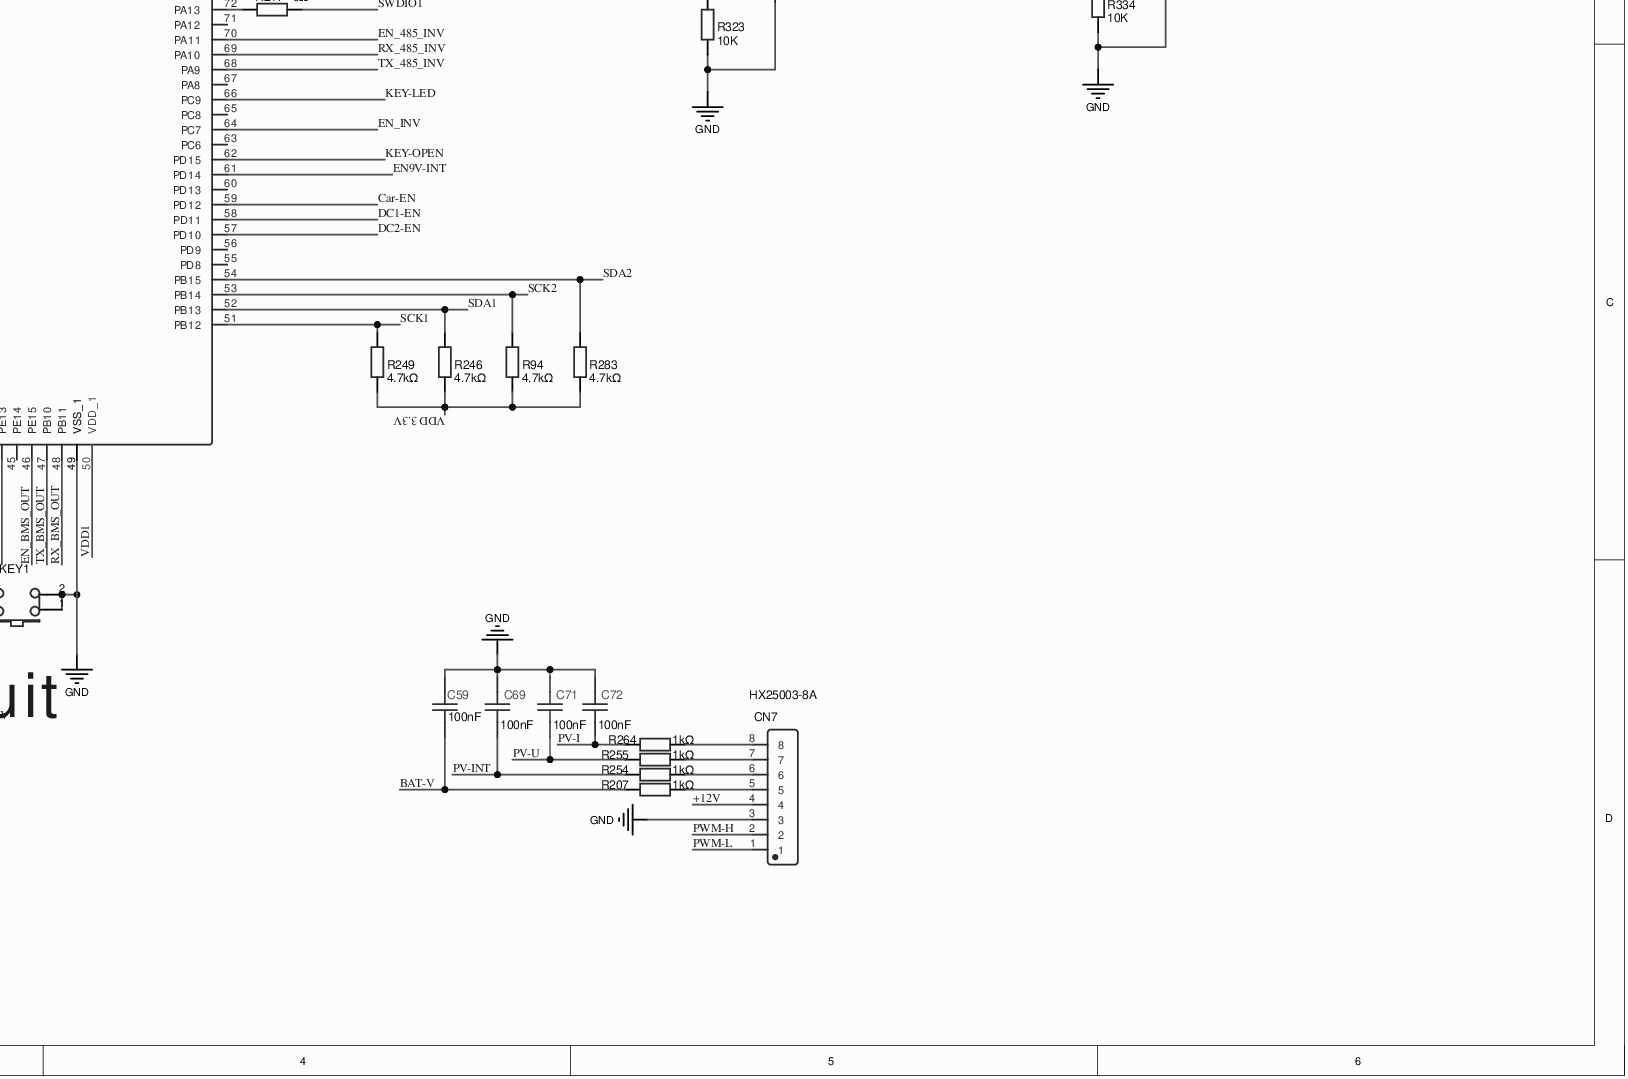
[diagram p0: MISC84402-7.SchDoc, bottom right]
# Altium project MISC84402-4.PrjPcb (part 2 of 7)
## Sheet MISC84402-7.SchDoc (continued)
### Parts (continued)
C9  100nF  [C0603]
C21  100nF  [C0603]
C26  100nF  [C0603]
C32  100nF  [C0603]
C34  100nF  [C0603]
C35  100nF  [C0603]
C39  1nF  [C0603]
C52  100nF  [C0603]
C59  100nF  [C0603]
C69  100nF  [C0603]
C71  100nF  [C0603]
C72  100nF  [C0603]
C73  100nF  [C0603]
C74  100nF  [C0603]
C76  220uF  [CAP-TH_BD6.3-P2.50-D1.0-FD]
C78  100nF  [C0603]
C85  100nF  [C0603]
C87  220uF  [CAP-TH_BD6.3-P2.50-D1.0-FD]
C94  220uF  [CAP-TH_BD6.3-P2.50-D1.0-FD]
C99  100nF  [C0603]
C100  100nF  [C0603]
C126  100nF  [C0603]
C127  100nF  [C0603]
C131  100nF  [C0603]
C133  100nF  [C0603]
C137  100nF  [C0603]
C149  20pF  [C0603]
C152  220uF  [CAP-TH_BD6.3-P2.50-D1.0-FD]
C156  220uF  [CAP-TH_BD6.3-P2.50-D1.0-FD]
C163  20pF  [C0603]
C164  20pF  [C0603]
C167  100nF  [C0603]
C178  4.7uF  [C0805]
CN2  HX25003-4A  [CONN-TH_4P-P2.50_HX25003-4A]
CN7  HX25003-8A  [CONN-TH_8P-P2.50_HX25003-8A]
CN10  HX25003-4A  [CONN-TH_4P-P2.50_HX25003-4A]
D14  SS12  [SMA_L4.3-W2.6-LS5.2-RD]
D46  SMAJ30  [SMA_L4.3-W2.5-LS5.0-BI]
D47  SMAJ30  [SMA_L4.3-W2.5-LS5.0-BI]
KEY1  4-1437565-2  [SW-SMD_4P-L6.0-W6.0-P4.50-LS8.6]  (value not drawn)
KEY2  4-1437565-2  [SW-SMD_4P-L6.0-W6.0-P4.50-LS8.6]  (value not drawn)
KEY3  4-1437565-2  [SW-SMD_4P-L6.0-W6.0-P4.50-LS8.6]  (value not drawn)
KEY4  4-1437565-2  [SW-SMD_4P-L6.0-W6.0-P4.50-LS8.6]  (value not drawn)
KEY5  4-1437565-2  [SW-SMD_4P-L6.0-W6.0-P4.50-LS8.6]  (value not drawn)
KEY7  4-1437565-2  [SW-SMD_4P-L6.0-W6.0-P4.50-LS8.6]  (value not drawn)
KEY8  4-1437565-2  [SW-SMD_4P-L6.0-W6.0-P4.50-LS8.6]  (value not drawn)
LED1  LED-0603_R  [LED0603_RED]  (value not drawn)
LED2  LED-0603_R  [LED0603_RED]  (value not drawn)
LED3  LED-0603_R  [LED0603_RED]  (value not drawn)
LED4  LED-0603_R  [LED0603_RED]  (value not drawn)
LED5  LED-0603_R  [LED0603_RED]  (value not drawn)
LED6  LED-0603_R  [LED0603_RED]  (value not drawn)
LED7  LED-0603_R  [LED0603_RED]  (value not drawn)
Q46  SS8050_C2898656  [SOT-23-3_L2.9-W1.3-P1.90-LS2.4-BR]
Q47  SS8050_C2898656  [SOT-23-3_L2.9-W1.3-P1.90-LS2.4-BR]
Q48  SS8050_C2898656  [SOT-23-3_L2.9-W1.3-P1.90-LS2.4-BR]
Q49  SS8050_C2898656  [SOT-23-3_L2.9-W1.3-P1.90-LS2.4-BR]
Q50  HSU4103  [TO-252-2_L6.6-W6.1-P4.57-LS9.9-BR]
Q51  SS8050_C2898656  [SOT-23-3_L2.9-W1.3-P1.90-LS2.4-BR]
Q54  SS8050_C2898656  [SOT-23-3_L2.9-W1.3-P1.90-LS2.4-BR]
R3  4.7kΩ  [R0603]
R33  100kΩ  [R0603]
R36  0Ω  [R0603]
R46  100kΩ  [R0603]
R47  1K  [R0603]
R57  100K  [NTC]
R64  2K  [R0603]
R78  2K  [R0603]
R79  2K  [R0603]
R80  0Ω  [R0603]
R86  1kΩ  [R0603]
R94  4.7kΩ  [R0603]
R118  2K  [R0603]
R150  10kΩ  [R0603]
R163  100K  [NTC]
R187  2K  [R0603]
R194  2K  [R0603]
R195  2K  [R0603]
R207  1kΩ  [R0603]
R217  0Ω  [R0603]
R219  4.7kΩ  [R0603]
R221  4.7kΩ  [R0603]
R222  0Ω  [R0603]
R224  5.1kΩ  [R0603]
R228  4.7kΩ  [R0603]
R237  0Ω  [R0603]
R246  4.7kΩ  [R0603]
R249  4.7kΩ  [R0603]
R250  4.7kΩ  [R0603]
R251  4.7kΩ  [R0603]
R252  4.7kΩ  [R0603]
R254  1kΩ  [R0603]
R255  1kΩ  [R0603]
R256  10Ω  [R0603]
R257  10Ω  [R0603]
R264  1kΩ  [R0603]
R269  470Ω  [R0603]
R280  1kΩ  [R0603]
R282  1kΩ  [R0603]
R283  4.7kΩ  [R0603]
R284  1kΩ  [R0603]
R285  1kΩ  [R0603]
R286  1kΩ  [R0603]
R293  100kΩ  [R0603]
R317  1kΩ  [R0603]
R323  10K  [R0603]
R324  1K  [R0603]
R325  2K  [R0603]
R332  10K  [R0603]
R333  2K  [R0603]
R334  10K  [R0603]
R335  2K  [R0603]
R336  10K  [R0603]
R337  2K  [R0603]
R338  0Ω  [R0603]
R348  0Ω  [R0603]
R349  5.1kΩ  [R0603]
R350  20K  [R0603]
R351  20K  [R0603]
R354  1kΩ  [R0603]
R355  1kΩ  [R0603]
R356  1kΩ  [R0603]
R363  2K  [R0603]
R364  2K  [R0603]
R365  10K  [R0603]
R366  4.7kΩ  [R0603]
U8  LM1117S-3.3  [SOT-223-3_L6.5-W3.4-P2.30-LS7.0-BR]
U13  GD32F103VCT6  [LQFP-100_L14.0-W14.0-P0.50-LS16.0-BL]
U14  LM1117S-3.3  [SOT-223-3_L6.5-W3.4-P2.30-LS7.0-BR]
U19  TL431_C2688223  [SOT-23-3_L2.9-W1.6-P1.90-LS2.8-BR-CW]
X1  8MHz  [HC-49S_L11.4-W4.8]

### Nets
GND: C5.2 C9.1 C21.1 C26.2 C32.1 C34.1 C35.1 C39.1 C52.2 C59.1 C69.1 C71.1 C72.1 C73.2 C74.2 C76.2 C78.1 C85.1 C87.2 C94.2 C99.1 C100.1 C126.1 C127.1 C131.1 C133.1 C137.1 C149.1 C152.2 C156.2 C163.1 C164.1 C167.2 C178.2 CN2.4 CN7.3 CN10.4 D46.1 D47.1 KEY1.1 KEY1.2 KEY2.3 KEY2.4 KEY3.1 KEY3.2 KEY4.1 KEY4.2 KEY5.3 KEY5.4 KEY7.3 KEY7.4 KEY8.3 KEY8.4 Q46.2(E) Q47.2(E) Q48.2(E) Q49.2(E) Q54.2(E) R57.1 R80.1 R163.2 R224.2 R323.2 R332.2 R334.2 R336.2 R338.1 R350.1 R365.2 U8.1(ADJ/GND) U13.10(VSS_5) U13.19(VSSA) U13.27(VSS_4) U13.49(VSS_1) U13.73(BOOT0) U13.74(VSS_2) U13.94(BOOT0) U13.99(VSS_3) U14.1(ADJ/GND) U19.2(ANODE)
2.5V: C39.2 R33.2 R46.2 R224.1 R269.1 U13.21(VREF+) U19.1(REF) U19.3(CATHODE)
13.6V-I: R317.2
13.6V-U: R86.2
+5V: C9.2 C76.1 C152.1 C167.1 Q50.2(S) R351.1 U14.3(IN)
+12V: CN7.4 CN10.3 LED1.1 LED2.1 LED3.1 LED4.1 LED5.1 LED6.1 LED7.1
BAT-V: C59.2 R207.1 U13.23(PA0_WAKEUP)
BUSY: U13.90(PB4)
Car-EN: U13.59(PD12)
Car-I: R356.2
DC1-EN: U13.58(PD11)
DC1-I: R354.2
DC2-EN: U13.57(PD10)
DC2-I: R355.2
EN9V-INT: U13.61(PD14)
EN_485_INV: U13.70(PA11)
EN_BMS_IN: U13.77(PA15)
EN_BMS_OUT: U13.46(PE15)
EN_INV: U13.64(PC7)
FAN1: U13.18(PC3)
FAN1-EN: U13.95(PB8)
FAN2: U13.43(PE12)
FAN2-EN: U13.96(PB9)
KEY9-EN: R364.1 U13.92(PB6)
KEY9-MCU: CN10.1 R366.1 U13.85(PD4)
KEY-DC: R337.1 U13.39(PE8)
KEY-LED: R325.1 U13.66(PC9)
KEY-OPEN: R333.1 U13.62(PD15)
KEY-USB: R335.1 U13.44(PE13)
LED-EN: U13.88(PD7)
MPPT-TEMP_TC: C127.2 R257.2 U13.16(PC1)
PC UART-RX: R47.1
PC UART-TX: R324.1
POW13.6-EN: U13.82(PD1)
POW24-EN: U13.81(PD0)
PV-I: C72.2 R264.1 U13.24(PA1)
PV-INT: C69.2 R150.1 R254.1 U13.3(PE4)
PV-U: C71.2 R255.1 U13.33(PC4)
PWM-H: CN7.2 U13.42(PE11)
PWM-L: CN7.1 U13.40(PE9)
RX_485_INV: U13.69(PA10)
RX_BMS_IN: U13.79(PC11)
RX_BMS_OUT: U13.48(PB11)
RXD-MODBUS: U13.86(PD5)
SCK1: R249.2 U13.51(PB12)
SCK2: R94.2 U13.53(PB14)
SDA1: R246.2 U13.52(PB13)
SDA2: R283.2 U13.54(PB15)
SWCLK1: CN2.3 R222.2
SWDIO1: CN2.1 R217.2
TEMP_TC: C126.2 R256.2 U13.15(PC0)
TX_485_INV: U13.68(PA9)
TX_BMS_IN: U13.78(PC10)
TX_BMS_OUT: U13.47(PB10)
TXD-MODBUS: U13.87(PD6)
USB-QC-I: R282.2
USB-QC-U1: R280.1
USB-QC-U2: R284.2
USB-QC-U3: R285.1
USB-QC-U4: R286.1
VCC9V: C78.2 C87.1 U8.3(IN)
VDD1: C131.2 C133.2 C137.2 C178.1 R36.2 R237.1 U13.11(VDD_5) U13.28(VDD_4) U13.50(VDD_1) U13.75(VDD_2) U13.100(VDD_3)
VDD5V: Q50.3(D)
VDD 3.3V: C32.2 C156.1 CN2.2 D14.1(K) R3.1 R36.1 R94.1 R150.2 R219.2 R221.2 R228.2 R246.1 R249.1 R250.2 R251.2 R252.2 R283.1 R293.2 R366.2 U14.2(OUT) U14.4(TAB)
VREF-EN: R269.2 U13.38(PE7)
NetC5_1: C5.1 R282.1 U13.26(PA3)
NetC21_2: C21.2 R354.1 U13.31(PA6)
NetC26_1: C26.1 R86.1 U13.29(PA4)
NetC34_2: C34.2 R317.1 U13.30(PA5)
NetC35_2: C35.2 R280.2 U13.25(PA2)
NetC52_1: C52.1 R284.1 U13.35(PB0)
NetC73_1: C73.1 R285.2 U13.36(PB1)
NetC74_1: C74.1 R286.2 U13.17(PC2)
NetC85_2: C85.2 C94.1 D14.2(A) U8.2(OUT) U8.4(TAB)
NetC99_2: C99.2 R355.1 U13.32(PA7)
NetC100_2: C100.2 R356.1 U13.34(PC5)
NetC149_2: C149.2 U13.13(OSC_OUT) X1.1(OSC1)
NetC163_2: C163.2 U13.12(OSC_IN) X1.2(OSC2)
NetC164_2: C164.2 R293.1 U13.14(NRST)
NetCN7_5: CN7.5 R207.2
NetCN7_6: CN7.6 R254.2
NetCN7_7: CN7.7 R255.2
NetCN7_8: CN7.8 R264.2
NetCN10_2: CN10.2 R363.1
NetD46_2: D46.2 R324.2 U13.80(PC12)
NetD47_2: D47.2 R47.2 U13.83(PD2)
NetKEY1_3: KEY1.3 KEY1.4 R3.2 U13.41(PE10)
NetKEY2_1: KEY2.1 KEY2.2 R252.1 U13.1(PE2)
NetKEY3_3: KEY3.3 KEY3.4 R251.1 U13.98(PE1)
NetKEY4_3: KEY4.3 KEY4.4 R250.1 U13.97(PE0)
NetKEY5_1: KEY5.1 KEY5.2 R221.1 U13.5(PE6)
NetKEY7_1: KEY7.1 KEY7.2 R228.1 U13.89(PB3)
NetKEY8_1: KEY8.1 KEY8.2 R219.1 U13.4(PE5)
NetLED1_2: LED1.2 R64.1
NetLED2_2: LED2.2 R78.1
NetLED3_2: LED3.2 R194.1
NetLED4_2: LED4.2 R195.1
NetLED5_2: LED5.2 R79.1
NetLED6_2: LED6.2 R118.1
NetLED7_2: LED7.2 R187.1
NetQ46_1: Q46.1(B) R323.1 R325.2
NetQ46_3: Q46.3(C) R64.2
NetQ47_1: Q47.1(B) R332.1 R333.2
NetQ47_3: Q47.3(C) R78.2 R79.2 R118.2 R187.2
NetQ48_1: Q48.1(B) R334.1 R335.2
NetQ48_3: Q48.3(C) R194.2
NetQ49_1: Q49.1(B) R336.1 R337.2
NetQ49_3: Q49.3(C) R195.2
NetQ50_1: Q50.1(G) R348.2 R351.2
NetQ51_1: Q51.1(B) R349.1 R350.2
NetQ51_2: Q51.2(E) R338.2
NetQ51_3: Q51.3(C) R348.1
NetQ54_1: Q54.1(B) R364.2 R365.1
NetQ54_3: Q54.3(C) R363.2
NetR33_1: R33.1 R57.2 R256.1
NetR46_1: R46.1 R163.1 R257.1
NetR80_2: R80.2 U13.20(VREF-)
NetR217_1: R217.1 U13.72(PA13)
NetR222_1: R222.1 U13.76(PA14)
NetR237_2: R237.2 U13.22(VDDA)
NetR349_2: R349.2 U13.84(PD3)

Not connected (* = marked no-connect by the designer): U13 2(PE3) 6(VBAT) 7(PC13_TAMPER_RTC) 8(PC14_OSC32_IN) 9(PC15_OSC32_OUT) 37(PB2) 45(PE14) 55(PD8) 56(PD9) 60(PD13) 63(PC6) 65(PC8) 67(PA8) 71(PA12) 91(PB5) 93(PB7)

### Notes on the sheet
- Near key6
- Near key7
- Near key5
- (near R64) Near key8
- MCU power supply and control circuit

### Library data of the parts
C5 C9 C21 C26 C32 C34 C35 C52 C59 C69 C71-C74 C78 C85 C99 C100 C126 C127 C131 C133 C137 C167 = 100nF: as C51 on sheet MISC84402-8; BOM_Supplier: LCSC; BOM_Supplier Part: C15725; BOM_JLCPCB Part Class: Extended Part; spicePre: C; spiceSymbolName: CL10B104KC8NNNC
C39 = 1nF: BOM_Manufacturer Part: CL10B102KB8NNNC; BOM_Manufacturer: SAMSUNG; nameAlias: Capacitance; BOM_Supplier: LCSC; BOM_Supplier Part: C1588; BOM_JLCPCB Part Class: Basic Part; spicePre: C; spiceSymbolName: CL10B102KB8NNNC
C76 C87 C94 C152 C156 = 220uF: BOM_Manufacturer: ValuePro; BOM_Manufacturer Part: 220uF 16V 6.3*11; nameAlias: Capacitance; BOM_Supplier: LCSC; BOM_Supplier Part: C43349; BOM_JLCPCB Part Class: Extended Part; spicePre: C; spiceSymbolName: 220uF 16V 6.3*11
C149 C163 C164 = 20pF: BOM_Manufacturer: YAGEO; BOM_Manufacturer Part: CC0603JRNPO9BN200; nameAlias: Capacitance; BOM_Supplier: LCSC; BOM_Supplier Part: C105621; BOM_JLCPCB Part Class: Extended Part; spicePre: C; spiceSymbolName: CC0603JRNPO9BN200
C178 = 4.7uF: BOM_Manufacturer Part: CL21A475KAQNNNE; BOM_Manufacturer: SAMSUNG; nameAlias: Capacitance; BOM_Supplier: LCSC; BOM_Supplier Part: C1779; BOM_JLCPCB Part Class: Basic Part; spicePre: C; spiceSymbolName: CL21A475KAQNNNE
CN2 CN10 = HX25003-4A: BOM_Manufacturer: HX(Zhejiang Yueqing Hongxing Elec); Contributor: LCSC; BOM_Supplier: LCSC; BOM_Supplier Part: C442301; BOM_Manufacturer Part: HX25003-4A; BOM_JLCPCB Part Class: Extended Part; spicePre: C; spiceSymbolName: HX25003-4A
CN7 = HX25003-8A: BOM_Manufacturer: HX(Zhejiang Yueqing Hongxing Elec); Contributor: LCSC; BOM_Supplier: LCSC; BOM_Supplier Part: C442305; BOM_Manufacturer Part: HX25003-8A; BOM_JLCPCB Part Class: Extended Part; spicePre: C; spiceSymbolName: HX25003-8A
D14 = SS12: BOM_Manufacturer: MDD; BOM_Supplier: LCSC; BOM_Manufacturer Part: SS12; BOM_Supplier Part: C2479; BOM_JLCPCB Part Class: Extended Part; spicePre: D; spiceSymbolName: SS12
D46 D47 = SMAJ30: BOM_Manufacturer: Shandong Jingdao Microelectronics; BOM_Manufacturer Part: SMAJ30CA; Contributor: LCSC; BOM_Supplier: LCSC; BOM_Supplier Part: C353455; BOM_JLCPCB Part Class: Extended Part; spicePre: D; spiceSymbolName: SMAJ30CA_C353455
KEY1-KEY5 KEY7 KEY8 = 4-1437565-2: BOM_Manufacturer: TE Connectivity; BOM_Supplier: LCSC; BOM_Manufacturer Part: 4-1437565-2; BOM_Supplier Part: C86487; BOM_JLCPCB Part Class: Extended Part; spicePre: K; spiceSymbolName: 4-1437565-2
LED1-LED7 = LED-0603_R: BOM_Manufacturer: EVERLIGHT (Taiwan); BOM_Manufacturer Part: 19-217/R6C-AL1M2VY/3T; Contributor: LCEDA_01; BOM_Supplier Part: C72044; BOM_Supplier: LCSC; spicePre: L; spiceSymbolName: LED-0603_R
Q46-Q49 Q51 Q54 = SS8050_C2898656: BOM_Manufacturer: YFW; BOM_Manufacturer Part: SS8050; Contributor: LCSC; BOM_Supplier: LCSC; BOM_Supplier Part: C2898656; spicePre: Q; spiceSymbolName: SS8050_C2898656
Q50 = HSU4103: BOM_Manufacturer: HUASHUO; Contributor: LCSC; BOM_Supplier: LCSC; BOM_Supplier Part: C508797; BOM_Manufacturer Part: HSU4103; BOM_JLCPCB Part Class: Extended Part; spicePre: Q; spiceSymbolName: HSU4103
R3 R94 R219 R221 R228 R246 R249-R252 R283 R366 = 4.7kΩ: BOM_Manufacturer: UniOhm; BOM_Manufacturer Part: 0603WAF4701T5E; nameAlias: Resistance; Resistance (Ohms): 4.7K; BOM_Supplier: LCSC; BOM_Supplier Part: C23162; BOM_JLCPCB Part Class: Basic Part; spicePre: R; spiceSymbolName: 0603WAF4701T5E
R33 R46 R293 = 100kΩ: BOM_Manufacturer: UniOhm; BOM_Manufacturer Part: 0603WAF1003T5E; nameAlias: Resistance; Resistance (Ohms): 100K; BOM_Supplier: LCSC; BOM_Supplier Part: C25803; BOM_JLCPCB Part Class: Basic Part; spicePre: R; spiceSymbolName: 0603WAF1003T5E
R36 R80 R217 R222 R237 R338 R348 = 0Ω: BOM_Manufacturer: UniOhm; BOM_Manufacturer Part: 0603WAF0000T5E; nameAlias: Resistance; Resistance (Ohms): 0; BOM_Supplier: LCSC; BOM_Supplier Part: C21189; BOM_JLCPCB Part Class: Basic Part; spicePre: R; spiceSymbolName: 0603WAF0000T5E
R47 R324 = 1K: as R67 on sheet MISC84402-8; BOM_Supplier: LCSC; BOM_Supplier Part: C73797; BOM_JLCPCB Part Class: Extended Part; spicePre: R; spiceSymbolName: RS-03K102JT
R57 R163 = 100K: BOM_Manufacturer: Sunlord; BOM_Manufacturer Part: SDNT1608X104F4250FTF; nameAlias: Value; BOM_Supplier: LCSC; BOM_Supplier Part: C95955; BOM_JLCPCB Part Class: Extended Part; spicePre: R; spiceSymbolName: SDNT1608X104F4250FTF
R64 R78 R79 R118 R187 R194 R195 R325 R333 R335 R337 R363 R364 = 2K: as R23 on sheet MISC84402-8; BOM_Supplier: LCSC; BOM_Supplier Part: C22975; BOM_JLCPCB Part Class: Basic Part; spicePre: R; spiceSymbolName: 0603WAF2001T5E
R86 R207 R254 R255 R264 R280 R282 R284-R286 R317 R354-R356 = 1kΩ: BOM_Manufacturer: UniOhm; BOM_Manufacturer Part: 0603WAF1001T5E; nameAlias: Resistance; Resistance (Ohms): 1K; BOM_Supplier: LCSC; BOM_Supplier Part: C21190; BOM_JLCPCB Part Class: Basic Part; spicePre: R; spiceSymbolName: 0603WAF1001T5E
R150 = 10kΩ: BOM_Manufacturer: UniOhm; BOM_Manufacturer Part: 0603WAF1002T5E; nameAlias: Resistance; Resistance (Ohms): 10K; BOM_Supplier: LCSC; BOM_Supplier Part: C25804; BOM_JLCPCB Part Class: Basic Part; spicePre: R; spiceSymbolName: 0603WAF1002T5E
R224 R349 = 5.1kΩ: BOM_Manufacturer Part: 0603WAF5101T5E; BOM_Manufacturer: UniOhm; Resistance (Ohms): 5.1K; nameAlias: Resistance; BOM_Supplier: LCSC; BOM_Supplier Part: C23186; BOM_JLCPCB Part Class: Basic Part; spicePre: R; spiceSymbolName: 0603WAF5101T5E
R256 R257 = 10Ω: BOM_Manufacturer: UniOhm; BOM_Manufacturer Part: 0603WAF100JT5E; nameAlias: Resistance; BOM_Supplier: LCSC; BOM_Supplier Part: C22859; Resistance (Ohms): 10Ω; BOM_JLCPCB Part Class: Basic Part; spicePre: R; spiceSymbolName: 0603WAF100JT5E
R269 = 470Ω: BOM_Manufacturer: UniOhm; BOM_Manufacturer Part: 0603WAF4700T5E; nameAlias: Resistance; Resistance (Ohms): 470; BOM_Supplier: LCSC; BOM_Supplier Part: C23179; BOM_JLCPCB Part Class: Basic Part; spicePre: R; spiceSymbolName: 0603WAF4700T5E
R323 R332 R334 R336 R365 = 10K: as R65 on sheet MISC84402-8; BOM_Supplier: LCSC; BOM_Supplier Part: C73797; spicePre: R; spiceSymbolName: RS-03K102JT
R350 R351 = 20K: BOM_Manufacturer: YAGEO; BOM_Manufacturer Part: RC0603FR-0720KL; nameAlias: Resistance (Ohms); Resistance: 20kΩ; BOM_Supplier: LCSC; BOM_Supplier Part: C105575; BOM_JLCPCB Part Class: Extended Part; spicePre: R; spiceSymbolName: RC0603FR-0720KL
U8 U14 = LM1117S-3.3: BOM_Manufacturer: HTC; BOM_Supplier: LCSC; BOM_Manufacturer Part: LM1117S-3.3; BOM_Supplier Part: C126027; BOM_JLCPCB Part Class: Extended Part; spicePre: U; spiceSymbolName: LM1117S-3.3
U13 = GD32F103VCT6: BOM_Manufacturer: GigaDevice; BOM_Supplier: LCSC; BOM_Manufacturer Part: GD32F103VCT6; BOM_Supplier Part: C77789; BOM_JLCPCB Part Class: Extended Part; spicePre: U; spiceSymbolName: GD32F103VCT6
U19 = TL431_C2688223: BOM_Manufacturer: WPMtek; BOM_Manufacturer Part: TL431; Contributor: LCSC; BOM_Supplier: LCSC; BOM_Supplier Part: C2688223; BOM_JLCPCB Part Class: Extended Part; spicePre: U; spiceSymbolName: TL431_C2688223
X1 = 8MHz: BOM_Manufacturer: YXC; BOM_Manufacturer Part: X49SM8MSD2SI; nameAlias: Frequency; BOM_Supplier: LCSC; BOM_Supplier Part: C106809; BOM_JLCPCB Part Class: Extended Part; spicePre: X; spiceSymbolName: X49SM8MSD2SI